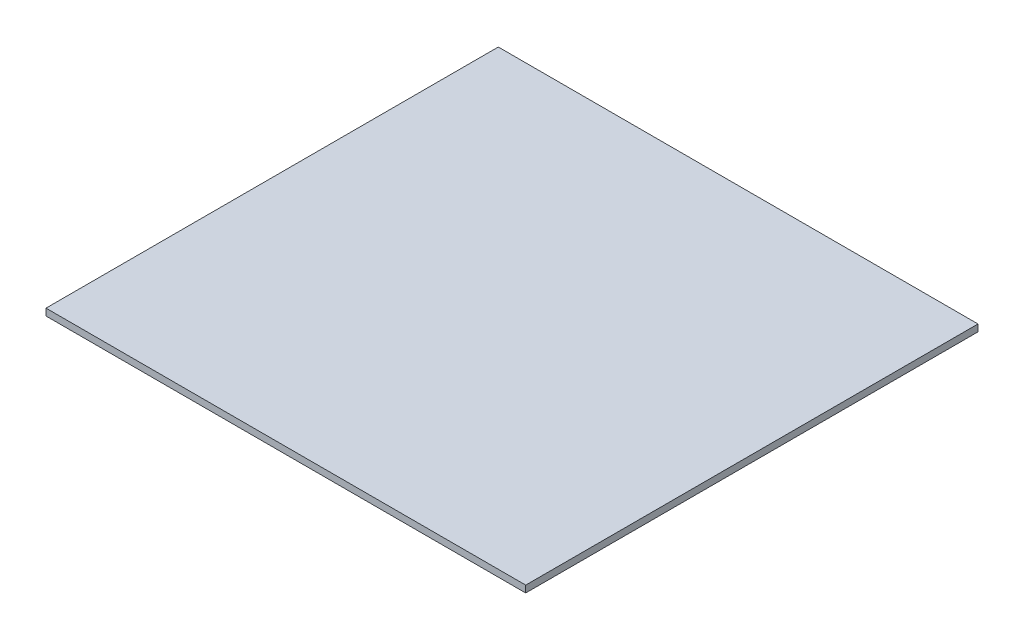
from build123d import *

# Parameters (mm, degrees)
SKETCH1_W           = 700
SKETCH1_H           = 660
BOSS_EXTRUDE1_DEPTH = 10


with BuildPart() as part:
    # Sketch1 → Boss-Extrude1 (new body)
    with BuildSketch(Plane(origin=(0, 0, 0), x_dir=(1, 0, 0), z_dir=(0, 1, 0))):
        Rectangle(SKETCH1_W, SKETCH1_H)
    extrude(amount=BOSS_EXTRUDE1_DEPTH)


solid = part.part
